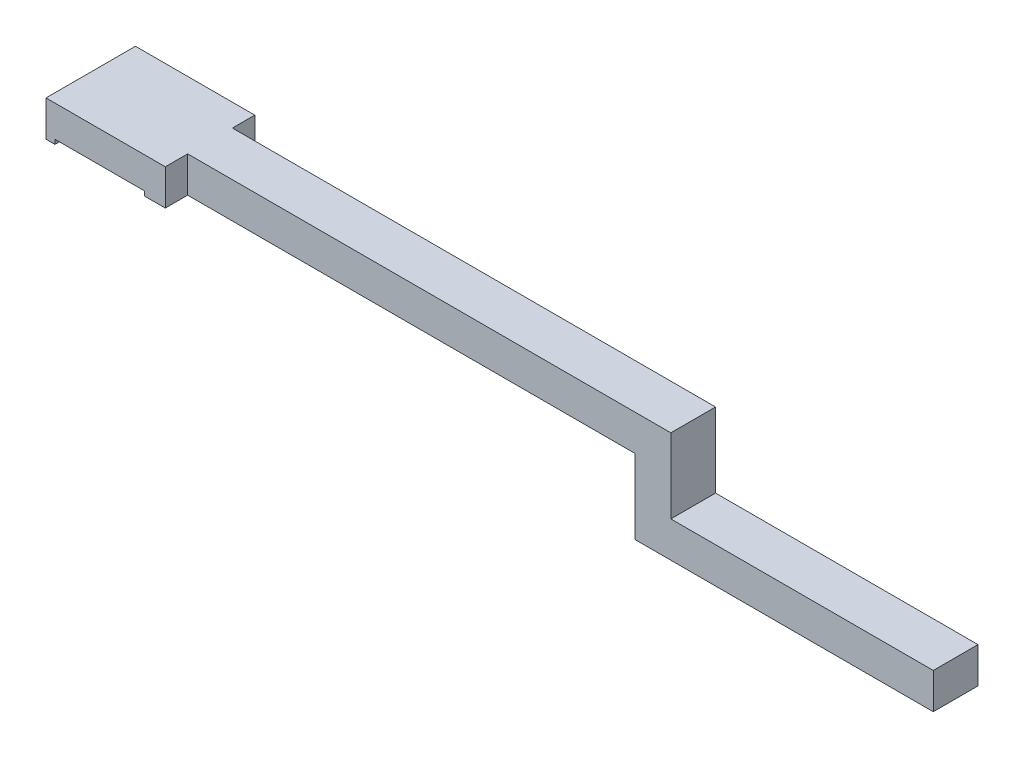
from build123d import *

# Parameters (mm, degrees)
EXTRUDE_5_DEPTH     = 7.5
SKETCH_7_W          = 40
SKETCH_7_H          = 30
EXTRUDE_6_DEPTH     = 12
SKETCH_8_W          = 30
SKETCH_8_H          = 30
CUT_EXTRUDE_1_DEPTH = 1.5


with BuildPart() as part:
    # 草图6 → 凸台-拉伸5 (new, symmetric)
    with BuildSketch(Plane.XY):
        Polygon((0, 0), (162, 0), (162, -25), (250, -25), (250, -37), (150, -37), (150, -12), (0, -12), align=None)
    extrude(amount=EXTRUDE_5_DEPTH, both=True)

    # 草图7 → 凸台-拉伸6 (add)
    with BuildSketch(Plane(origin=(0, 0, 0), x_dir=(1, 0, 0), z_dir=(0, 1, 0))):
        with Locations((-20, 0)):
            Rectangle(SKETCH_7_W, SKETCH_7_H)
    extrude(amount=-EXTRUDE_6_DEPTH)

    # 草图8 → 切除-拉伸1 (cut)
    with BuildSketch(Plane(origin=(0, -12, 0), x_dir=(1, 0, 0), z_dir=(0, 1, 0))):
        with Locations((-22, 0)):
            Rectangle(SKETCH_8_W, SKETCH_8_H)
    extrude(amount=CUT_EXTRUDE_1_DEPTH, mode=Mode.SUBTRACT)


solid = part.part
